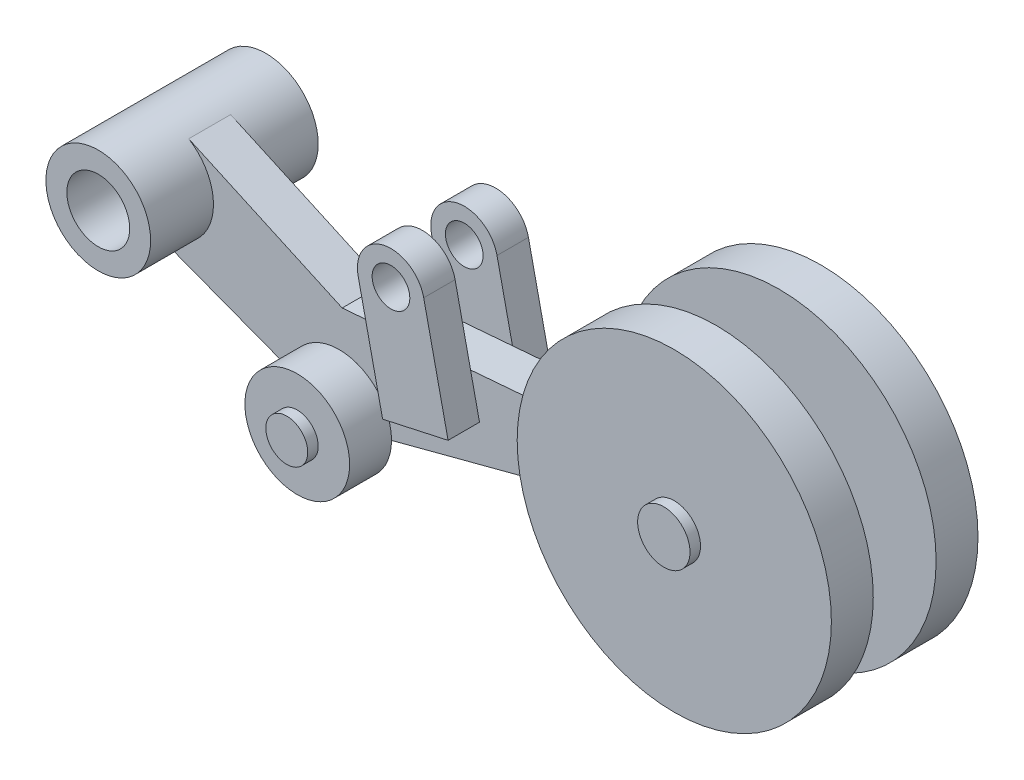
from build123d import *

# Parameters (mm, degrees)
EXTRUDE_1_DEPTH      = 40
EXTRUDE_1_DEPTH_BACK = 40
SKETCH_1_R           = 25
SKETCH_1_R_2         = 15
EXTRUDE_2_DEPTH      = 10
EXTRUDE_2_DEPTH_BACK = 10
SKETCH_3_R           = 12.5
SKETCH_3_R_2         = 10
EXTRUDE_3_DEPTH      = 30
SKETCH_4_R           = 25
SKETCH_4_R_2         = 75
BOSS_EXTRUDE4_DEPTH  = 20
SKETCH_5_R           = 9
BOSS_EXTRUDE5_DEPTH  = 15


with BuildPart() as part:
    # 草图1 → 凸台-拉伸1 (new, two sides: drawn at the far end of the back side and taken through both)
    with BuildSketch(Plane.XY.offset(-EXTRUDE_1_DEPTH_BACK)):
        Circle(SKETCH_1_R)
        Circle(SKETCH_1_R_2, mode=Mode.SUBTRACT)
    extrude(amount=EXTRUDE_1_DEPTH + EXTRUDE_1_DEPTH_BACK)

    # 草图2 → 凸台-拉伸2 (add, two sides: drawn at the far end of the back side and taken through both)
    with BuildSketch(Plane.XY.offset(-EXTRUDE_2_DEPTH_BACK)):
        with BuildLine():
            Line((-11.804411719, -22.037601139), (86.449952125, -59.348644826))
            ThreePointArc((86.449952125, -59.348644826), (89.473468939, -59.986128631), (92.547259147, -59.670132928))
            Line((92.547259147, -59.670132928), (273.184073933, -12.08766616))
            ThreePointArc((273.184073933, -12.08766616), (282.19931165, 2.725214721), (267.737534205, 12.293544994))
            Line((267.737534205, 12.293544994), (174.388702716, -4.886083694))
            Line((174.388702716, -4.886083694), (86.450111626, -12.08766616))
            Line((86.450111626, -12.08766616), (7.341932544, 23.897615499))
            ThreePointArc((7.341932544, 23.897615499), (20.013015277, -8.341662634), (-11.804411719, -22.037601139))
        make_face()
    extrude(amount=EXTRUDE_2_DEPTH + EXTRUDE_2_DEPTH_BACK)

    # 草图3 → 凸台-拉伸3 (add)
    with BuildSketch(Plane.XY.offset(10)):
        with Locations((270, 0)):
            Circle(SKETCH_3_R)
        with Locations((90, -50)):
            Circle(SKETCH_3_R_2)
    extrude(amount=EXTRUDE_3_DEPTH)

    # 草图4 → Boss-Extrude4 (add)
    with BuildSketch(Plane.XY.offset(15)):
        with Locations((90, -50)):
            Circle(SKETCH_4_R)
        with Locations((270, 0)):
            Circle(SKETCH_4_R_2)
    extrude(amount=BOSS_EXTRUDE4_DEPTH)

    # 草图5 → Boss-Extrude5 (add)
    with BuildSketch(Plane.XY.offset(10)):
        with BuildLine():
            Line((120.752986945, -33.386484264), (109.111101455, 19.729618285))
            ThreePointArc((109.111101455, 19.729618285), (121.314568975, 38.784155291), (140.36910598, 26.58068777))
            Line((140.36910598, 26.58068777), (152.010991471, -26.535414779))
            Line((152.010991471, -26.535414779), (120.752986945, -33.386484264))
        make_face()
        with Locations((124.740103717, 23.155153028)):
            Circle(SKETCH_5_R, mode=Mode.SUBTRACT)
    extrude(amount=BOSS_EXTRUDE5_DEPTH)

    # Mirror2: part across plane


with BuildPart() as part_1:
    add(part.part)
    add(part.part.mirror(Plane.XY))


solid = part_1.part
